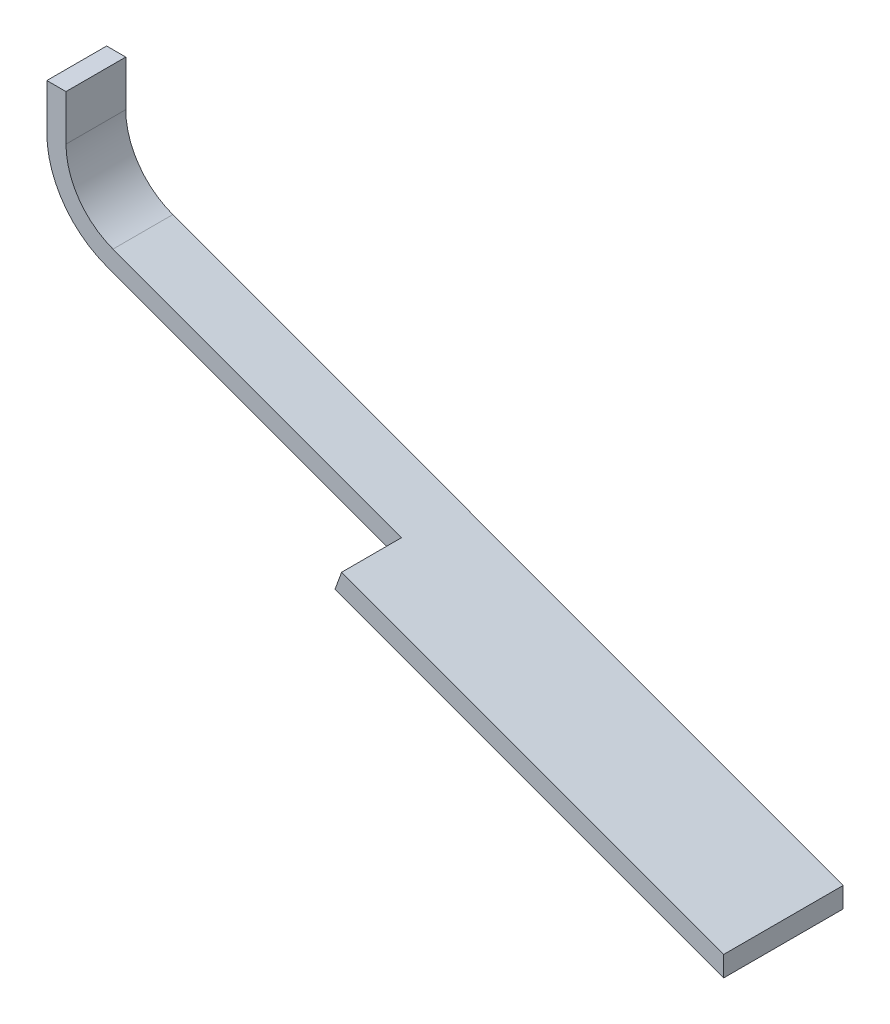
from build123d import *

# Parameters (mm, degrees)
EXTRUDE_1_DEPTH     = 50
SKETCH_2_W          = 128.455604429
SKETCH_2_H          = 25
SKETCH_2_W_2        = 42.23428711
CUT_EXTRUDE_1_DEPTH = 49


with BuildPart() as part:
    # 草图1 → 凸台-拉伸1 (new body)
    with BuildSketch(Plane.XY):
        with BuildLine():
            Line((-158.499845276, 75.499845276), (-158.499845276, 56.452935893))
            ThreePointArc((-158.499845276, 56.452935893), (-151.653526546, 34.694072336), (-133.581521944, 20.77563589))
            Line((-133.581521944, 20.77563589), (146.746117531, -82.011165251))
            Line((146.746117531, -82.011165251), (149.500154724, -83.020978889))
            Line((149.500154724, -83.020978889), (149.500154724, -74.500154724))
            Line((149.500154724, -74.500154724), (-130.827484751, 28.286646417))
            ThreePointArc((-130.827484751, 28.286646417), (-145.094856805, 39.274885717), (-150.499845276, 56.452935893))
            Line((-150.499845276, 56.452935893), (-150.499845276, 75.499845276))
            Line((-150.499845276, 75.499845276), (-158.499845276, 75.499845276))
        make_face()
    extrude(amount=EXTRUDE_1_DEPTH)

    # 草图2 → 切除-拉伸1 (cut)
    with BuildSketch(Plane(origin=(-9.115968963, -24.861733537, 0), x_dir=(0.9388763158866098, -0.3442546491584201, 0), z_dir=(-0.3442546491584201, -0.9388763158866098, 0))):
        with Locations((-68.340834223, 37.5)):
            Rectangle(SKETCH_2_W, SKETCH_2_H)
        with Locations((-153.685779993, 37.5)):
            Rectangle(SKETCH_2_W_2, SKETCH_2_H)
    extrude(amount=-CUT_EXTRUDE_1_DEPTH, mode=Mode.SUBTRACT)


solid = part.part
